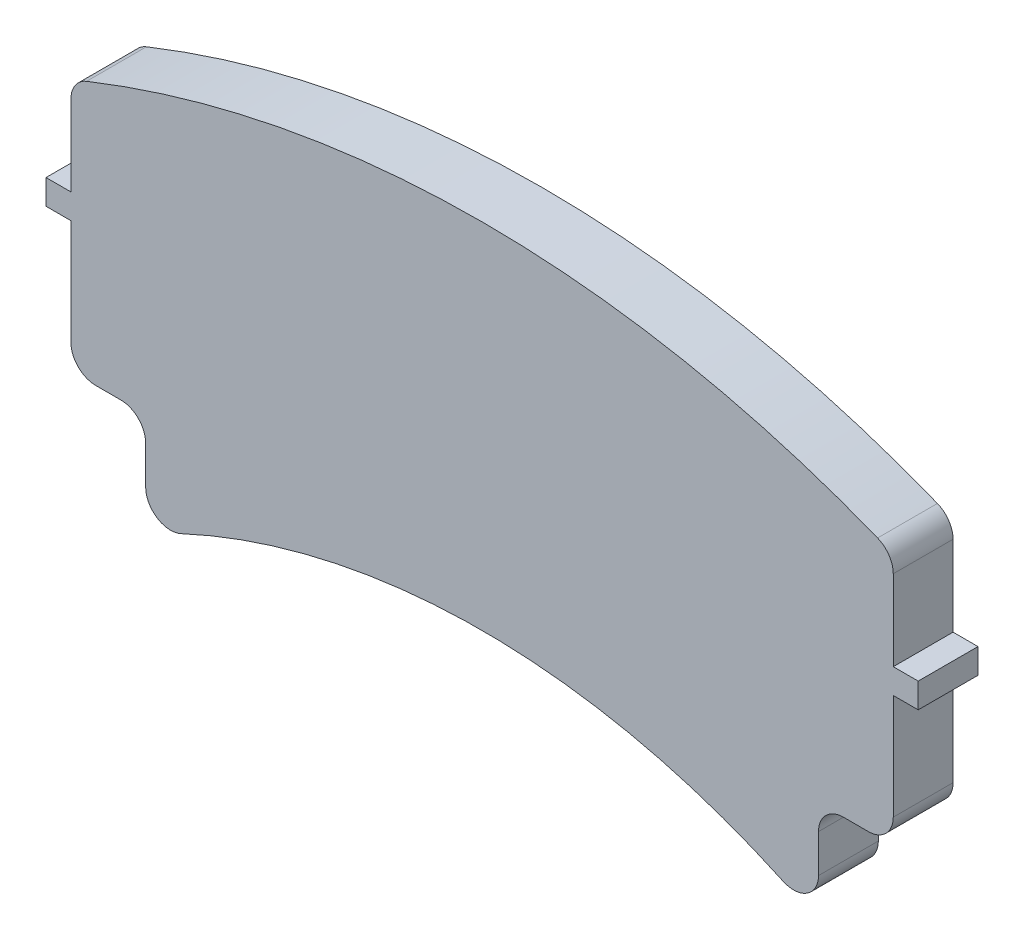
from build123d import *

# Parameters (mm, degrees)
BOSS_EXTRUDE1_DEPTH = 6
SKETCH2_W           = 15
SKETCH2_H           = 30
CUT_EXTRUDE1_DEPTH  = 30
FILLET2_R           = 5
SKETCH3_W           = 5
SKETCH3_H           = 5
BOSS_EXTRUDE2_DEPTH = 12


with BuildPart() as part:
    # Sketch1 → Boss-Extrude1 (new, symmetric)
    with BuildSketch(Plane.XY):
        with BuildLine():
            Line((-82.5, 197.45822343), (-82.5, 116.802183199))
            ThreePointArc((-82.5, 116.802183199), (0, 143), (82.5, 116.802183199))
            Line((82.5, 116.802183199), (82.5, 197.45822343))
            ThreePointArc((82.5, 197.45822343), (0, 214), (-82.5, 197.45822343))
        make_face()
    extrude(amount=BOSS_EXTRUDE1_DEPTH, both=True)

    # Sketch2 → Cut-Extrude1 (cut)
    with BuildSketch(Plane.XY.offset(6)):
        with Locations((-75, 131.802183199)):
            Rectangle(SKETCH2_W, SKETCH2_H)
        with Locations((75, 131.802183199)):
            Rectangle(SKETCH2_W, SKETCH2_H)
    extrude(amount=-CUT_EXTRUDE1_DEPTH, mode=Mode.SUBTRACT)

    # Fillet2
    fillet2_edges = [part.edges().sort_by_distance(p)[0] for p in [
        (-82.5, 146.802183199, 0),
        (-67.5, 126.066450731, 0),
        (-67.5, 146.802183199, 0),
        (82.5, 146.802183199, 0),
        (67.5, 126.066450731, 0),
        (67.5, 146.802183199, 0),
        (-82.5, 197.45822343, 0),
        (82.5, 197.45822343, 0),
    ]]
    fillet(fillet2_edges, radius=FILLET2_R)

    # Sketch3 → Boss-Extrude2 (add)
    with BuildSketch(Plane.XY.offset(6)):
        with Locations((85, 175.45101432)):
            Rectangle(SKETCH3_W, SKETCH3_H)
        with Locations((-85, 175.45101432)):
            Rectangle(SKETCH3_W, SKETCH3_H)
    extrude(amount=-BOSS_EXTRUDE2_DEPTH)


solid = part.part
